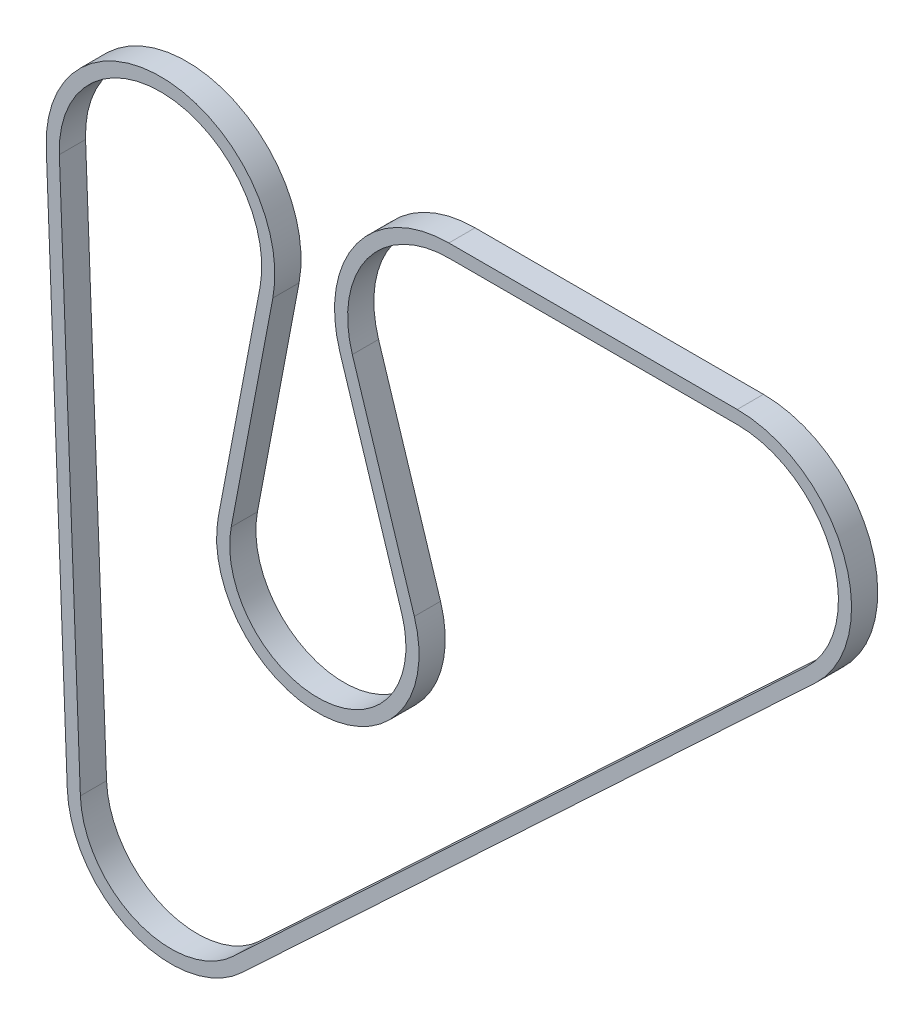
from build123d import *

# Parameters (mm, degrees)
EXTRUDE_1_DEPTH = 10


with BuildPart() as part:
    # 草图2 → 拉伸-薄壁1 (new body)
    with BuildSketch(Plane.XY):
        with BuildLine():
            Line((245.832281676, 176.176927505), (27.081748613, -28.88898874))
            ThreePointArc((27.081748613, -28.88898874), (-15.038455107, -36.631129472), (-39.568477007, -1.526566661))
            Line((-39.568477007, -1.526566661), (-47.587213234, 206.31838899))
            ThreePointArc((-47.587213234, 206.31838899), (-0.748703771, 251.498299345), (38.852898358, 199.857391364))
            Line((38.852898358, 199.857391364), (22.971322702, 116.275878645))
            ThreePointArc((22.971322702, 116.275878645), (57.994709331, 76.439587045), (88.052734333, 120.144081921))
            Line((88.052734333, 120.144081921), (64.413334144, 194.838609646))
            ThreePointArc((64.413334144, 194.838609646), (70.809318853, 233.773803242), (106, 251.619639764))
            Line((106, 251.619639764), (216, 251.619639764))
            ThreePointArc((216, 251.619639764), (256.563431385, 224.039981525), (245.832281676, 176.176927505))
        make_face()
        with BuildLine():
            Line((242.412688823, 179.824719264), (23.66215576, -25.241196981))
            ThreePointArc((23.66215576, -25.241196981), (-13.139560233, -32.00574319), (-34.572193971, -1.333808191))
            Line((-34.572193971, -1.333808191), (-42.590930198, 206.511147461))
            ThreePointArc((-42.590930198, 206.511147461), (-1.121390965, 246.512208266), (33.940787828, 200.790756321))
            Line((33.940787828, 200.790756321), (18.059212172, 117.209243602))
            ThreePointArc((18.059212172, 117.209243602), (58.291367675, 71.448395421), (92.819700095, 121.652736099))
            Line((92.819700095, 121.652736099), (69.180299905, 196.347263824))
            ThreePointArc((69.180299905, 196.347263824), (74.843130382, 230.819422671), (106, 246.619639764))
            Line((106, 246.619639764), (216, 246.619639764))
            ThreePointArc((216, 246.619639764), (251.913756192, 222.201362315), (242.412688823, 179.824719264))
        make_face(mode=Mode.SUBTRACT)
    extrude(amount=EXTRUDE_1_DEPTH)


solid = part.part
